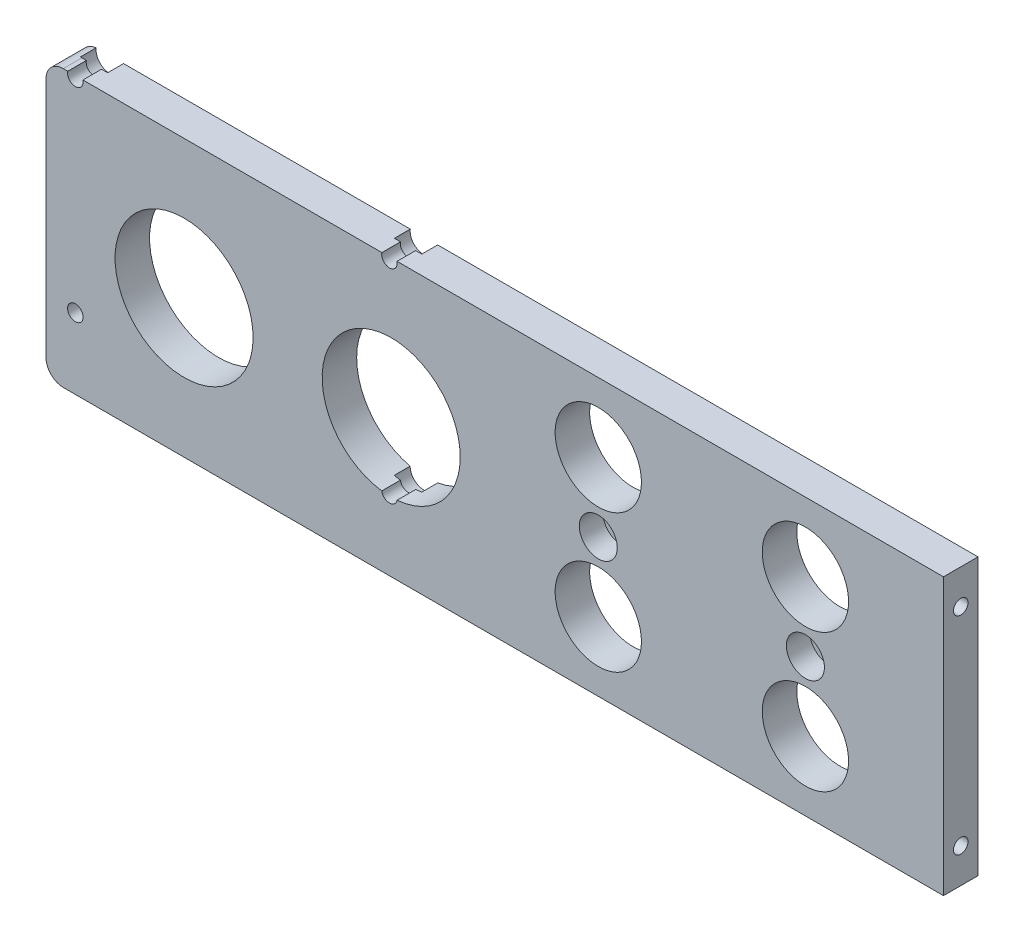
from build123d import *

# Parameters (mm, degrees)
SKETCH_1_W                = 260
SKETCH_1_H                = 80
EXTRUDE_1_DEPTH           = 10
CUT_EXTRUDE_1_REACH       = 138.382
SKETCH_2_R                = 20
CUT_EXTRUDE_2_REACH       = 138.382
SKETCH_3_R                = 12.5
HOLE_WIZARD_M5_1_D        = 4.2
HOLE_WIZARD_M5_1_DEPTH    = 12.4
HOLE_WIZARD_M5_1_TIP      = 1.2618073
HOLE_WIZARD_1_D           = 6.6
HOLE_WIZARD_1_CBORE_D     = 11
HOLE_WIZARD_1_CBORE_DEPTH = 6.8
HOLE_WIZARD_2_D           = 4.5
HOLE_WIZARD_2_DEPTH       = 10
HOLE_WIZARD_2_CBORE_D     = 8
HOLE_WIZARD_2_CBORE_DEPTH = 4.6
FILLET_1_R                = 5


with BuildPart() as part:
    # 草图1 → 凸台-拉伸1 (new body)
    with BuildSketch(Plane.XY):
        Rectangle(SKETCH_1_W, SKETCH_1_H)
    extrude(amount=EXTRUDE_1_DEPTH)

    # 草图2 → 切除-拉伸1 (cut, up to next)
    with BuildSketch(Plane.XY.offset(10), mode=Mode.PRIVATE) as cut_extrude_1_sk1:
        with Locations((-90, 0)):
            Circle(SKETCH_2_R)
    cut_extrude_1_tool1 = extrude(cut_extrude_1_sk1.sketch, amount=-CUT_EXTRUDE_1_REACH, mode=Mode.PRIVATE) & part.part
    # 草图2 → 切除-拉伸1 (cut, up to next)
    with BuildSketch(Plane.XY.offset(10), mode=Mode.PRIVATE) as cut_extrude_1_sk2:
        with Locations((-30, 0)):
            Circle(SKETCH_2_R)
    cut_extrude_1_tool2 = extrude(cut_extrude_1_sk2.sketch, amount=-CUT_EXTRUDE_1_REACH, mode=Mode.PRIVATE) & part.part
    add(cut_extrude_1_tool1.solids().sort_by_distance((-90, 0, 10))[0], mode=Mode.SUBTRACT)
    add(cut_extrude_1_tool2.solids().sort_by_distance((-30, 0, 10))[0], mode=Mode.SUBTRACT)

    # 草图3 → 切除-拉伸2 (cut, up to next)
    with BuildSketch(Plane.XY.offset(10), mode=Mode.PRIVATE) as cut_extrude_2_sk1:
        with Locations((30, -20)):
            Circle(SKETCH_3_R)
    cut_extrude_2_tool1 = extrude(cut_extrude_2_sk1.sketch, amount=-CUT_EXTRUDE_2_REACH, mode=Mode.PRIVATE) & part.part
    # 草图3 → 切除-拉伸2 (cut, up to next)
    with BuildSketch(Plane.XY.offset(10), mode=Mode.PRIVATE) as cut_extrude_2_sk2:
        with Locations((90, -20)):
            Circle(SKETCH_3_R)
    cut_extrude_2_tool2 = extrude(cut_extrude_2_sk2.sketch, amount=-CUT_EXTRUDE_2_REACH, mode=Mode.PRIVATE) & part.part
    # 草图3 → 切除-拉伸2 (cut, up to next)
    with BuildSketch(Plane.XY.offset(10), mode=Mode.PRIVATE) as cut_extrude_2_sk3:
        with Locations((30, 20)):
            Circle(SKETCH_3_R)
    cut_extrude_2_tool3 = extrude(cut_extrude_2_sk3.sketch, amount=-CUT_EXTRUDE_2_REACH, mode=Mode.PRIVATE) & part.part
    # 草图3 → 切除-拉伸2 (cut, up to next)
    with BuildSketch(Plane.XY.offset(10), mode=Mode.PRIVATE) as cut_extrude_2_sk4:
        with Locations((90, 20)):
            Circle(SKETCH_3_R)
    cut_extrude_2_tool4 = extrude(cut_extrude_2_sk4.sketch, amount=-CUT_EXTRUDE_2_REACH, mode=Mode.PRIVATE) & part.part
    add(cut_extrude_2_tool1.solids().sort_by_distance((30, -20, 10))[0], mode=Mode.SUBTRACT)
    add(cut_extrude_2_tool2.solids().sort_by_distance((90, -20, 10))[0], mode=Mode.SUBTRACT)
    add(cut_extrude_2_tool3.solids().sort_by_distance((30, 20, 10))[0], mode=Mode.SUBTRACT)
    add(cut_extrude_2_tool4.solids().sort_by_distance((90, 20, 10))[0], mode=Mode.SUBTRACT)

    # M5 螺纹孔1
    with Locations(Plane(origin=(130, 0, 0), x_dir=(0, 0, -1), z_dir=(1, 0, 0))):
        with Locations((-5, 30), (-5, -30)):
            Hole(HOLE_WIZARD_M5_1_D / 2, depth=HOLE_WIZARD_M5_1_DEPTH)
            with Locations((0, 0, -(HOLE_WIZARD_M5_1_DEPTH + HOLE_WIZARD_M5_1_TIP / 2))):  # 118° drill point
                Cone(0, HOLE_WIZARD_M5_1_D / 2, HOLE_WIZARD_M5_1_TIP, mode=Mode.SUBTRACT)

    # 打孔尺寸(%根据)内六角圆柱头螺钉的类型1 (through all)
    with Locations(Plane.XY.offset(10)):
        with Locations((90, 0), (30, 0)):
            CounterBoreHole(HOLE_WIZARD_1_D / 2, HOLE_WIZARD_1_CBORE_D / 2, HOLE_WIZARD_1_CBORE_DEPTH)

    # 打孔尺寸(%根据)内六角圆柱头螺钉的类型2
    with Locations(Plane(origin=(0, 0, 0), x_dir=(-1, 0, 0), z_dir=(0, 0, -1))):
        with Locations((30.500000316, -19.5), (30.500000316, 39.5), (121.500000316, 39.5), (121.500000316, -19.5)):
            CounterBoreHole(HOLE_WIZARD_2_D / 2, HOLE_WIZARD_2_CBORE_D / 2, HOLE_WIZARD_2_CBORE_DEPTH, depth=HOLE_WIZARD_2_DEPTH)

    # 圆角1
    fillet_1_edges = [part.edges().sort_by_distance(p)[0] for p in [
        (-130, 40, 5),
        (-130, -40, 5),
    ]]
    fillet(fillet_1_edges, radius=FILLET_1_R)


solid = part.part
